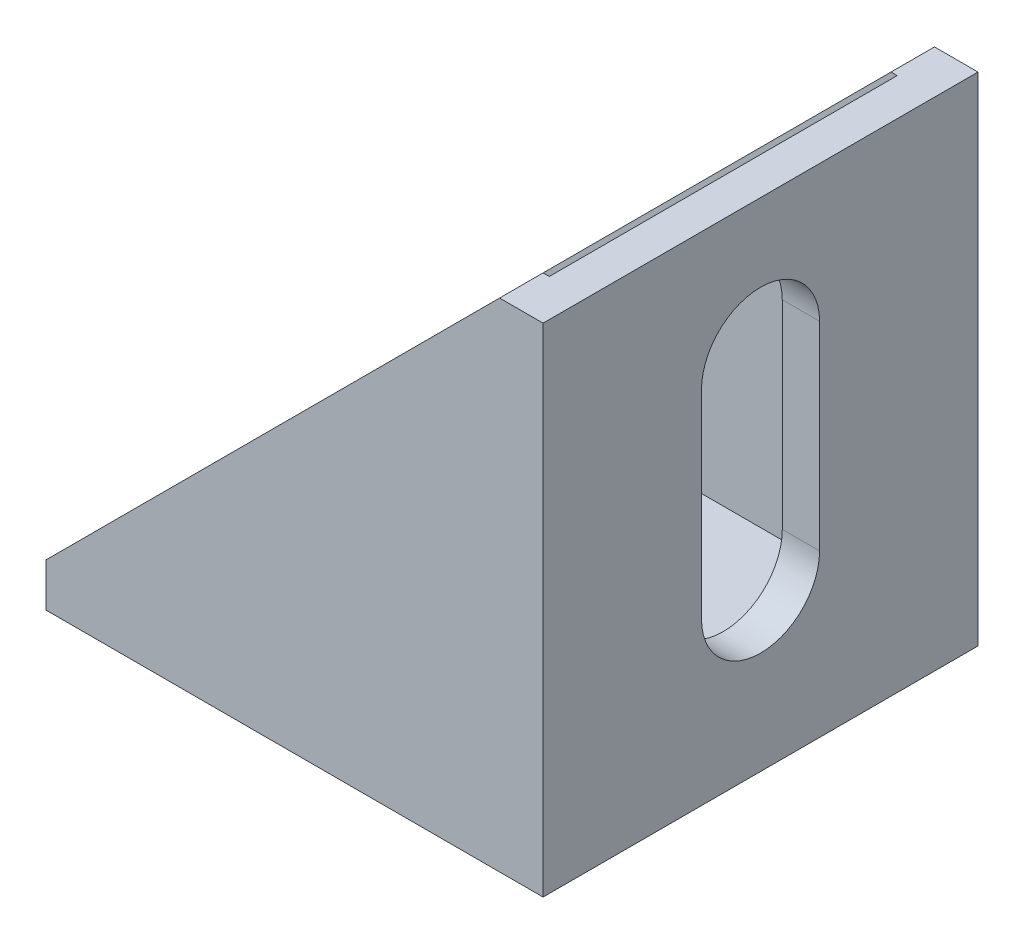
from build123d import *

# Parameters (mm, degrees)
EXTRUDE_1_DEPTH     = 17.5
CUT_EXTRUDE_1_DEPTH = 14
CUT_EXTRUDE_2_DEPTH = 47.706530593
CUT_EXTRUDE_3_DEPTH = 58.22979993


with BuildPart() as part:
    # 草图1 → 凸台-拉伸1 (new, symmetric)
    with BuildSketch(Plane.XY):
        Polygon((-22.5, 0), (-22.5, 3.5), (14, 40), (17.5, 40), (17.5, 0), align=None)
    extrude(amount=EXTRUDE_1_DEPTH, both=True)

    # 草图2 → 切除-拉伸1 (cut, symmetric)
    with BuildSketch(Plane.XY):
        Polygon((14.5, 3), (14.5, 49.29015486), (-34.195136802, 3), align=None)
    extrude(amount=CUT_EXTRUDE_1_DEPTH, both=True, mode=Mode.SUBTRACT)

    # 草图4 → 切除-拉伸2 (cut, through all)
    with BuildSketch(Plane(origin=(0, 3, 0), x_dir=(1, 0, 0), z_dir=(0, 1, 0))):
        with BuildLine():
            Line((-11.5, 4.75), (4.5, 4.75))
            ThreePointArc((4.5, 4.75), (9.25, 0), (4.5, -4.75))
            Line((4.5, -4.75), (-11.5, -4.75))
            ThreePointArc((-11.5, -4.75), (-16.25, 0), (-11.5, 4.75))
        make_face()
    extrude(amount=-CUT_EXTRUDE_2_DEPTH, mode=Mode.SUBTRACT)

    # 草图5 → 切除-拉伸3 (cut, through all)
    with BuildSketch(Plane.ZY.offset(-14.5)):
        with BuildLine():
            Line((-4.75, 13), (-4.75, 29))
            ThreePointArc((-4.75, 29), (0, 33.75), (4.75, 29))
            Line((4.75, 29), (4.75, 13))
            ThreePointArc((4.75, 13), (0, 8.25), (-4.75, 13))
        make_face()
    extrude(amount=-CUT_EXTRUDE_3_DEPTH, mode=Mode.SUBTRACT)


solid = part.part
